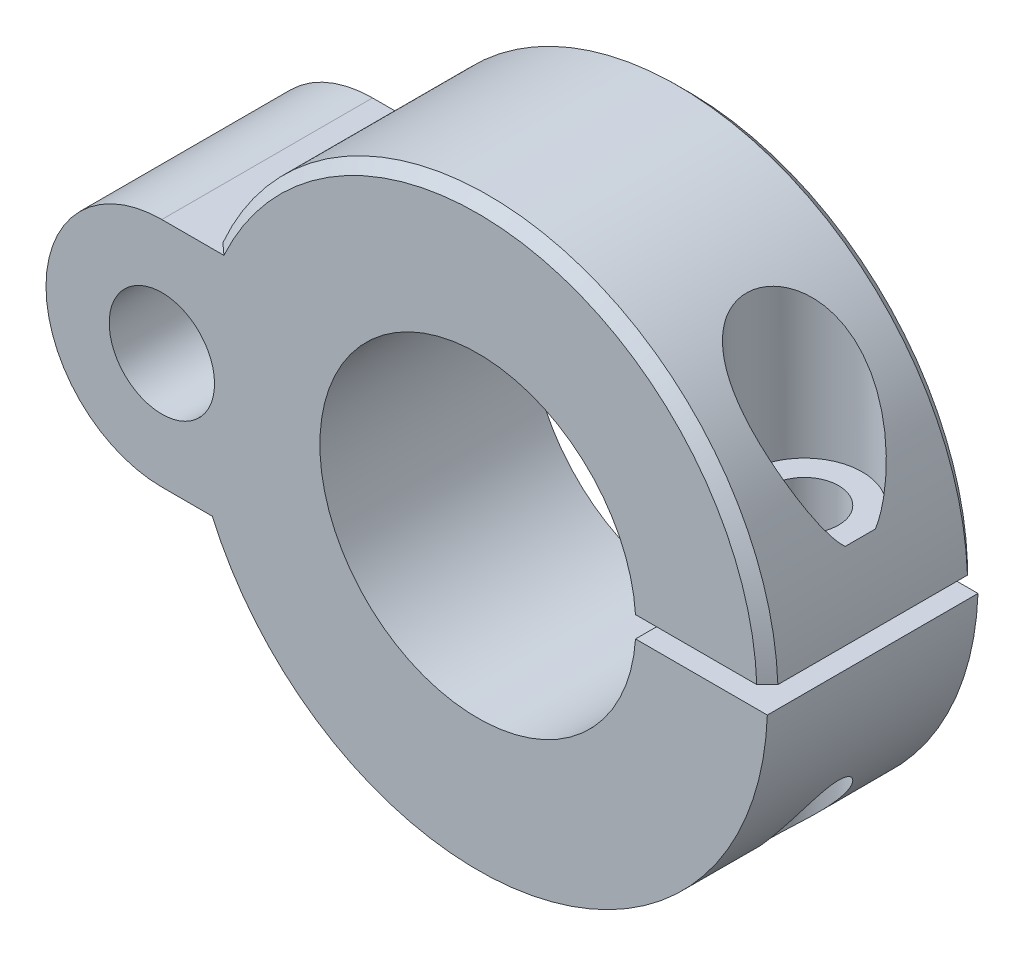
from build123d import *

# Parameters (mm, degrees)
EXTRUDE_1_DEPTH              = 20
CUT_EXTRUDE_1_DEPTH          = 54.265842714
SKETCH_3_W                   = 15
SKETCH_3_H                   = 20
HOLE_WIZARD_10_0_10_1_D      = 10
SKETCH_6_W                   = 2.5
SKETCH_6_H                   = 26.5
HOLE_WIZARD_M6_1_D           = 6.5
HOLE_WIZARD_M6_1_DEPTH       = 50.215633411
HOLE_WIZARD_M6_1_CBORE_D     = 11
HOLE_WIZARD_M6_1_CBORE_DEPTH = 14.715633411
CHAMFER_1_SIZE               = 1


with BuildPart() as part:
    # 草图1 → 凸台-拉伸1 (new body)
    with BuildSketch(Plane.XY.offset(10)):
        with BuildLine():
            Line((-25.204166322, 11), (-30, 11))
            ThreePointArc((-30, 11), (-41, 0), (-30, -11))
            Line((-30, -11), (-25.204166322, -11))
            ThreePointArc((-25.204166322, -11), (27.5, 0), (-25.204166322, 11))
        make_face()
    extrude(amount=-EXTRUDE_1_DEPTH)

    # 草图2 → 切除-拉伸1 (cut, through all)
    with BuildSketch(Plane(origin=(0, 0, -10), x_dir=(-1, 0, 0), z_dir=(0, 0, -1))):
        with BuildLine():
            Line((-27.481812167, -1), (-14.966629547, -1))
            ThreePointArc((-14.966629547, -1), (-15, 0), (-14.966629547, 1))
            Line((-14.966629547, 1), (-27.481812167, 1))
            ThreePointArc((-27.481812167, 1), (-27.5, 0), (-27.481812167, -1))
        make_face()
    extrude(amount=-CUT_EXTRUDE_1_DEPTH, mode=Mode.SUBTRACT)

    # 草图3 → 切除-旋转1 (revolve, cut)
    with BuildSketch(Plane.XZ):
        with Locations((7.5, 0)):
            Rectangle(SKETCH_3_W, SKETCH_3_H)
    revolve(axis=Axis((0, 0, 10), (0, 0, -1)), mode=Mode.SUBTRACT)

    # Ø10.0 (10) 直径孔1 (through all)
    with Locations(Plane.XY.offset(10)):
        with Locations((-30, 0)):
            Hole(HOLE_WIZARD_10_0_10_1_D / 2)

    # 草图6 → Ø5.0 (5) 直径孔1 (revolve, cut)
    with BuildSketch(Plane(origin=(21, -1, 0), x_dir=(0, 0, 1), z_dir=(1, 0, 0))):
        with Locations((1.25, 13.25)):
            Rectangle(SKETCH_6_W, SKETCH_6_H)
    revolve(axis=Axis((21, 5.35, 0), (0, -1, 0)), mode=Mode.SUBTRACT)

    # M6 六角头螺栓的柱形沉头孔1
    with Locations(Plane(origin=(0, 22.715633411, 0), x_dir=(1, 0, 0), z_dir=(0, 1, 0))):
        with Locations((21, 0)):
            CounterBoreHole(HOLE_WIZARD_M6_1_D / 2, HOLE_WIZARD_M6_1_CBORE_D / 2, HOLE_WIZARD_M6_1_CBORE_DEPTH, depth=HOLE_WIZARD_M6_1_DEPTH)

    # 倒角1
    chamfer_1_edges = [part.edges().sort_by_distance(p)[0] for p in [
        (5.128052033, 27.017643908, -10),
        (5.128052033, 27.017643908, 10),
    ]]
    chamfer(chamfer_1_edges, length=CHAMFER_1_SIZE)


solid = part.part
